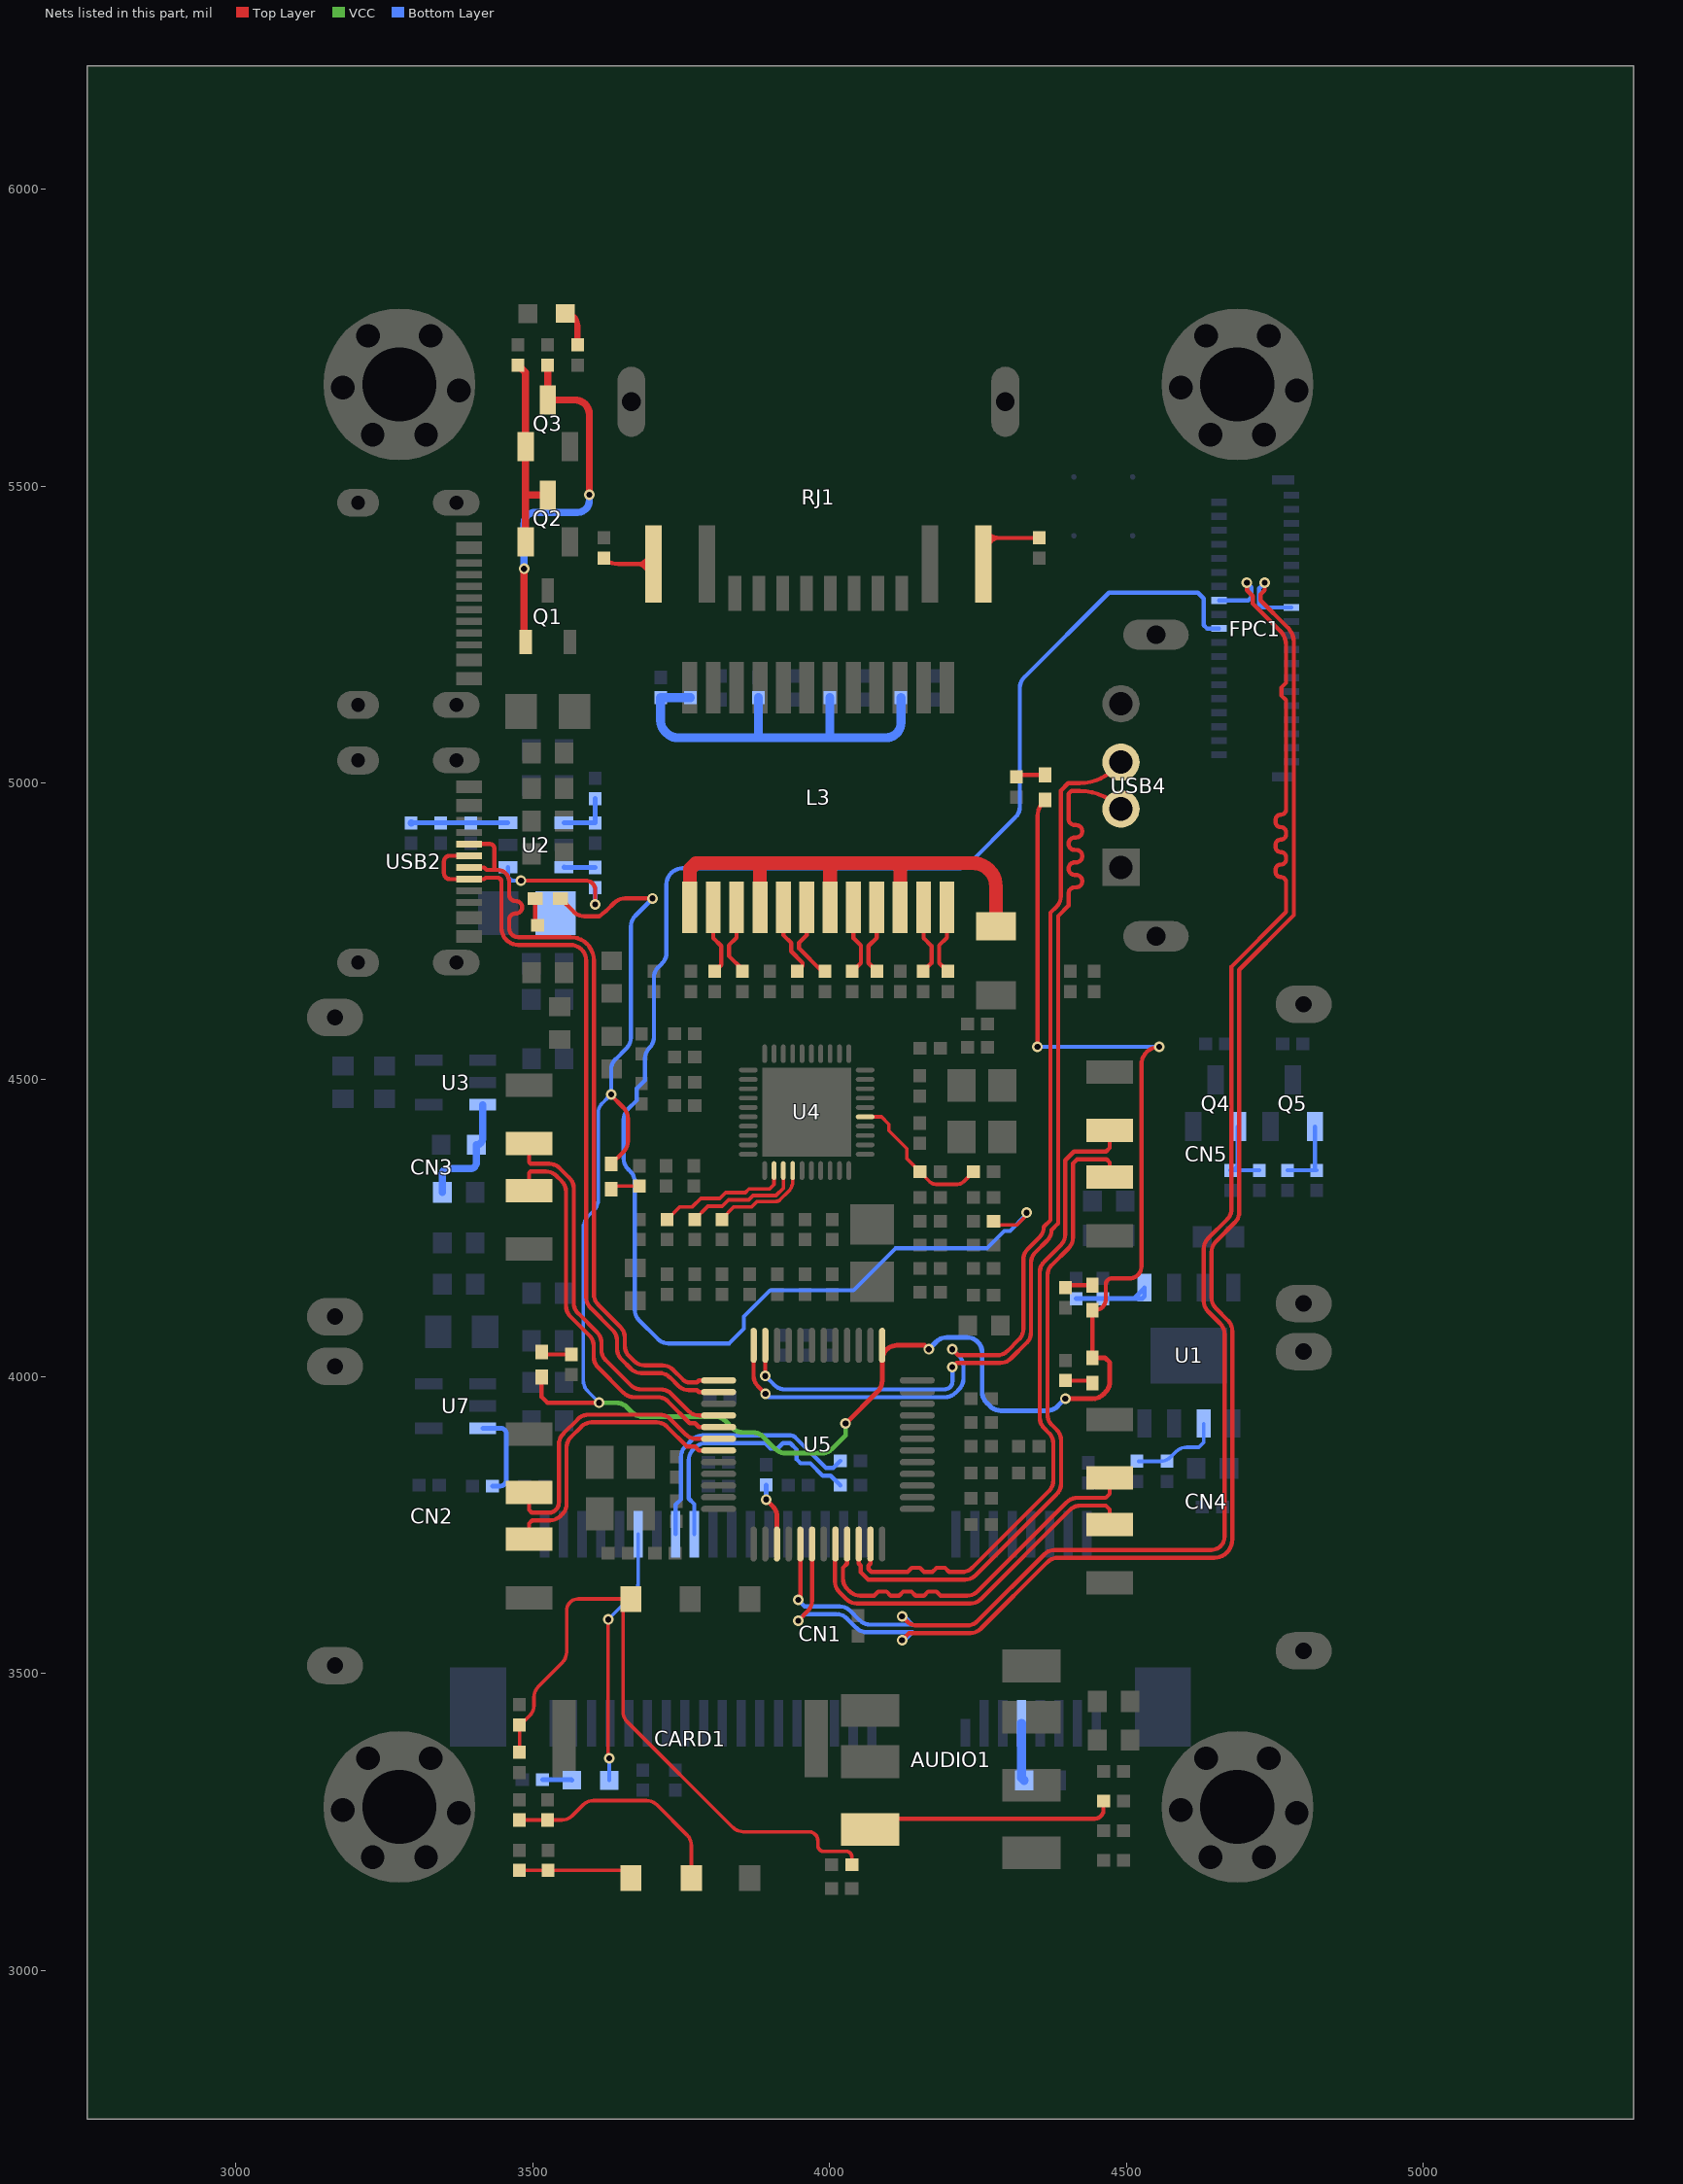
[diagram p0: the nets of this part, all layers, seen from the top]
# Altium PCB MISC84334.PcbDoc (part 4 of 8)
Units mil, origin at the board's own origin, x right, y up, seen from the top; angles counter-clockwise.
Board outline 2605.13 x 3457.4 mil, 4 copper layers (Top Layer, GND, VCC, Bottom Layer), stack 62.447 mil thick; 209 components, 149 nets, 735 pads, 529 vias.

## Via types
v1: diameter 18, hole 10, Top Layer to Bottom Layer, 529 vias

## Nets (pads, with @x,y where several pads share a name; then routed paths per layer and width w, separated by ;. In a path a pad name is that pad's centre, name@x,y a point inside that pad or via, vN(x,y) a via of type N, cw(c..) or ccw(c..) an arc to the next point about the centre after c; other vN are vias at no path point) (continued)
$2N2798: R45.1 U4.24 | length 168.6
  Top Layer w6: R45.1@3819.38,4264.89 3819.38,4266.28 3839.29,4286.19 3869.29,4286.19 3878.29,4295.19 3910.05,4295.19 ccw(c3910.05,4305.08) 3917.04,4298.09 3930.84,4311.88 ccw(c3913.16,4329.56) 3938.16,4329.56 U4.24@3938.16,4347.19
$2N2799: R46.1 U4.23 | length 200.8
  Top Layer w6: R46.1@3772.99,4264.89 3795.29,4287.19 3819.29,4287.19 3830,4297.9 3864,4297.9 3871.29,4305.19 3910.01,4305.19 3922.36,4317.54 U4.23@3922.36,4347.19
$2N2800: R48.1 U4.22 | length 228.1
  Top Layer w6: R48.1@3726.52,4264.89 3726.99,4264.89 3748.29,4286.19 3769.29,4286.19 3783.29,4300.19 3815.29,4300.19 3825.29,4310.19 3858.29,4310.19 3864.29,4316.19 3899.29,4316.19 3906.66,4323.56 U4.22@3906.66,4347.19
$2N2814: R23.1 R28.1 U4.35 | length 253.3
  Top Layer w6: U4.35@4060.16,4437.69 4087.79,4437.69 4100.29,4425.19 4100.29,4414.32 4130.29,4384.32 4130.29,4367.24 4169.11,4328.43 ccw(c4179.58,4338.9) 4179.58,4324.09 4215.64,4324.09 ccw(c4215.64,4338.35) 4225.73,4328.27 R23.1@4242.55,4345.09
$2N6665: R51.2 RJ1.12 | length 177.4
  Top Layer w7: RJ1.12@4259.39,5368.57 4259.39,5412.63 4285.36,5412.63 ; RJ1.12@4267.36,5420.09 ccw(c4285.36,5438.09) 4285.36,5412.63 ; RJ1.12@4268.79,5403.48 4272.7,5407.39 cw(c4285.36,5394.74) 4285.36,5412.63 ; R51.2@4353.17,5412.63 4285.36,5412.63
$2N6719: R47.2 RJ1.9 | length 132.6
  Top Layer w7: R47.2@3620.13,5378.55 ccw(c3644.22,5402.64) 3644.22,5368.57 3678.43,5368.57 ; RJ1.9@3695.84,5356.12 3686.9,5365.06 ccw(c3678.43,5356.58) 3678.43,5368.57 ; RJ1.9@3697.91,5382.25 3688.34,5372.68 cw(c3678.43,5382.59) 3678.43,5368.57 ; RJ1.9@3703.49,5368.57 3678.43,5368.57
$2N7042: C21.2 R37.1 R38.1 R39.1 R40.1 | length 701.2
  Bottom Layer w8: 3880.59,5076.51 3880.91,5076.19 ; 4000.59,5076.38 4000.78,5076.19
  Bottom Layer w15: R40.1@3765.59,5143.55 C21.2@3715.59,5143.55 3715.59,5104.69 ccw(c3740.59,5104.69) 3722.91,5087.01 3726.41,5083.51 ccw(c3744.09,5101.19) 3744.09,5076.19 3880.91,5076.19 4000.78,5076.19 4095.65,5076.19 ccw(c4095.65,5101.13) 4120.59,5101.13 R37.1@4120.59,5143.55 ; 3880.59,5076.51 R39.1@3880.59,5143.55 ; 4000.59,5076.38 R38.1@4000.59,5143.55
$2N7674: L3.2 R24.2 | length 118
  Top Layer w7: L3.2@3804.27,4790.55 3804.27,4738.76 3817.7,4725.34 3817.7,4693.42 R24.2@3806.91,4682.63
$2N7677: L3.3 R25.2 | length 122.6
  Top Layer w7: L3.3@3843.64,4790.55 3843.64,4739.38 3830.7,4726.44 3830.7,4708.65 3853.28,4686.07 R25.2@3853.28,4682.63
$2N7680: L3.5 R27.2 | length 125.2
  Top Layer w7: L3.5@3922.39,4790.55 3922.39,4743.74 3935.58,4730.56 3935.58,4716.36 3955.08,4696.85 3955.08,4691.69 R27.2@3946.02,4682.63
$2N7683: L3.6 R29.2 | length 134.1
  Top Layer w7: L3.6@3961.76,4790.55 3961.76,4743.74 3948.74,4730.72 3948.74,4721.58 3987.69,4682.63 R29.2@3992.38,4682.63
$2N7686: L3.8 R31.2 | length 118.9
  Top Layer w7: R31.2@4038.75,4682.63 4052.94,4696.81 4052.94,4726.33 4040.5,4738.76 L3.8@4040.5,4790.55
$2N7689: L3.9 R32.2 | length 119.6
  Top Layer w7: L3.9@4079.86,4790.55 4079.87,4739.38 4065.94,4725.45 4065.94,4696.81 R32.2@4080.12,4682.63
$2N7692: L3.12 R35.2 | length 119.2
  Top Layer w7: L3.12@4197.98,4790.55 4197.98,4739.38 4185.04,4726.44 4185.04,4696.81 R35.2@4199.22,4682.63
$2N7695: L3.11 R34.2 | length 119.4
  Top Layer w7: R34.2@4157.86,4682.63 4172.04,4696.81 4172.04,4725.34 4158.61,4738.76 L3.11@4158.61,4790.55
$2N7873: C20.2 L3.1 L3.4 L3.7 L3.10 | length 897.6
  Top Layer w15: 4000.66,4865.19 4001.13,4864.72 ; 4119.15,4865.19 4119.23,4865.11
  Top Layer w23: L3.1@3764.9,4790.55 3764.9,4854.8 3775.29,4865.19 3883.24,4865.19 ; L3.4@3883.02,4790.55 3883.02,4864.97 3883.24,4865.19 ; L3.7@4001.13,4790.55 4001.13,4864.72 ; 4119.15,4865.19 4000.66,4865.19 3883.24,4865.19 ; L3.10@4119.23,4790.55 4119.23,4865.11 4240.81,4865.11 cw(c4240.81,4825.33) 4280.59,4825.33 C20.2@4280.59,4758.81
$3N2816: CN1.42 LED8.1 | length 435.4
  Top Layer w6: v1(3627.29,3591.19) 3627.29,3358.95 v1(3629.05,3357.19)
  Bottom Layer w6: v1(3627.29,3591.19) 3670.54,3634.44 ccw(c3652.87,3652.12) 3677.87,3652.12 CN1.42@3677.87,3735.04 ; LED8.1@3629.05,3320.24 v1(3629.05,3357.19)
$3N2817: LED8.2 R70.1 | length 49.6
  Bottom Layer w8: R70.1@3516.74,3321.19 3565.42,3321.19 LED8.2@3566.1,3320.51
$3N2819: CN1.9 L7.2 | length 97.8
  Bottom Layer w15: CN1.9@4323.54,3416.14 4323.54,3324.73 L7.2@4328.04,3320.23
$3N2827: CN1.36 R68.1 | length 445.9
  Bottom Layer w7: CN1.36@3772.36,3735.04 3772.36,3785.64 3763.11,3794.89 3763.11,3859.65 cw(c3788.11,3859.65) 3770.43,3877.33 3773.97,3880.87 cw(c3791.65,3863.19) 3791.65,3888.19 3891.63,3888.19 3900.63,3879.19 3912.63,3879.19 3921.63,3888.19 3933.91,3888.19 3944.87,3877.23 3944.87,3860.61 3951.41,3854.07 3968.03,3854.07 3988.71,3833.38 4002.06,3833.38 R68.1@4018.25,3817.19
$3N2828: CN1.38 R69.1 | length 448
  Bottom Layer w7: CN1.38@3740.86,3735.04 3740.86,3784.51 3750.11,3793.76 3750.11,3865.04 cw(c3775.11,3865.04) 3757.43,3882.71 3768.58,3893.87 cw(c3786.26,3876.19) 3786.26,3901.19 3934.44,3901.19 cw(c3934.44,3889.47) 3942.72,3897.76 3994.1,3846.38 4006.44,3846.38 R69.1@4018.25,3858.19
$3N3897: CARD1.C2 D6.1 R63.2 | length 391.6
  Top Layer w6: R63.2@3477.77,3253.55 D6.1@3525.59,3253.55 3549.3,3253.55 ccw(c3549.3,3278.55) 3566.97,3260.87 3584.97,3278.87 cw(c3602.65,3261.19) 3602.65,3286.19 3691.94,3286.19 cw(c3691.94,3261.19) 3709.61,3278.87 3760.27,3228.21 cw(c3742.6,3210.53) 3767.6,3210.53 CARD1.C2@3767.6,3155.36
$3N3904: CARD1.C3 D5.1 R64.2 | length 193
  Top Layer w6: R64.2@3478.09,3168.55 D5.1@3525.8,3168.55 3652.4,3168.55 CARD1.C3@3665.6,3155.36
$3N4163: CARD1.C7 D8.1 R62.1 R65.1 | length 1097.8
  Top Layer w6: D8.1@3478.04,3367.63 R65.1@3478.04,3413.55 3479.65,3413.55 3494.97,3428.87 ccw(c3477.29,3446.55) 3502.29,3446.55 3502.29,3460.38 cw(c3527.29,3460.38) 3509.61,3478.06 3549.97,3518.41 ccw(c3532.29,3536.09) 3557.29,3536.09 3557.29,3606.19 cw(c3576.93,3606.19) 3576.93,3625.83 CARD1.C7@3665.6,3625.83 3652.29,3612.52 3652.29,3436.55 ccw(c3677.29,3436.55) 3659.61,3418.87 3837.47,3241.01 ccw(c3855.15,3258.69) 3855.15,3233.69 3965.41,3233.69 cw(c3965.41,3218.51) 3980.59,3218.51 3980.59,3210.59 ccw(c3990.59,3210.59) 3990.59,3200.59 4028.68,3200.59 cw(c4028.68,3191.5) 4037.77,3191.5 R62.1@4037.77,3177.96
$3N6344: C57.2 Q4.1 R66.2 | length 129.5
  Bottom Layer w7: Q4.1@4687.99,4421.22 4687.99,4360.03 cw(c4675.59,4360.03) R66.2@4675.59,4347.63 C57.2@4724.41,4347.63
$3N6376: C58.1 Q5.1 R72.1 | length 123.9
  Bottom Layer w7: R72.1@4771.77,4347.63 C58.1@4820.59,4347.63 cw(c4820.59,4350.23) 4817.99,4350.23 Q5.1@4817.99,4421.22
$4N635: AUDIO1.6 R75.2 | length 434.5
  Top Layer w7: AUDIO1.6@4068.8,3237.48 4068.8,3255.59 4446.61,3255.59 ccw(c4446.61,3270.59) 4461.61,3270.59 R75.2@4461.61,3285.59
$5N539: Q1.1 Q3.3 R6.2 | length 620.4
  Top Layer w12: v1(3485.59,5360.59) 3485.59,5239.83 Q1.1@3488.19,5237.23 ; R6.2@3525.59,5703.55 Q3.3@3525.59,5644.96 3571.22,5644.96 cw(c3571.22,5620.59) 3595.59,5620.59 v1(3595.59,5485.59)
  Bottom Layer w12: v1(3485.59,5360.59) 3485.59,5437.16 cw(c3504.02,5437.16) 3504.02,5455.59 3575.59,5455.59 ccw(c3575.59,5475.59) 3595.59,5475.59 v1(3595.59,5485.59)
$5N540: Q2.1 Q2.3 Q3.1 R5.2 | length 340.3
  Top Layer w12: R5.2@3475.59,5703.55 3488.19,5690.95 Q3.1@3488.19,5566.22 3488.19,5485.5 ; Q2.1@3488.19,5406.12 3488.19,5485.5 ; Q2.3@3525.59,5484.86 3488.82,5484.86 3488.19,5485.5
$5N1057: R2.1 R3.2 U1.5 | length 156.7
  Bottom Layer w8: R3.2@4415.59,4131.5 R2.1@4460.59,4131.5 4512.66,4131.5 ; U1.5@4530.59,4150.09 U1.5@4530.59,4149.43 ; 4512.66,4131.5 U1.5@4530.59,4149.43 ; 4512.66,4131.5 4526.8,4131.5 4530.59,4135.29 U1.5@4530.59,4149.43
$5N1555: R1.1 R4.2 U1.2 | length 152.6
  Bottom Layer w6: R4.2@4520.59,3857.63 4557.38,3857.63 ccw(c4557.38,3882.63) 4575.05,3864.95 4583.97,3873.87 cw(c4601.65,3856.19) 4601.65,3881.19 4622.29,3881.19 4630.59,3889.49 U1.2@4630.59,3921.09
$5N2255: R7.1 R9.2 U2.4 | length 93.6
  Bottom Layer w8: U2.4@3552.84,4932.99 R7.1@3605.23,4932.99 ; R7.1@3605.59,4932.63 R7.1@3605.23,4932.99 ; R9.2@3605.59,4973.55 3605.59,4933.35 R7.1@3605.23,4932.99
$5N2259: C6.2 U2.1 | length 227.3
  Top Layer w7: v1(3480.59,4835.59) 3589.34,4835.59 cw(c3589.34,4819.34) 3605.59,4819.34 v1(3605.59,4795.59)
  Bottom Layer w7: U2.1@3458.35,4858.19 3458.35,4844.68 ccw(c3467.43,4844.68) 3467.43,4835.59 v1(3480.59,4835.59) v1@3480.59,4835.95
  Bottom Layer w8: v1(3605.59,4795.59) C6.2@3605.59,4823.55
$5N2260: C6.1 L1.1 U2.6 | length 53.1
  Bottom Layer w8: U2.6@3552.84,4858.19 ccw(c3553.4,4858.19) 3553.4,4857.63 C6.1@3605.59,4857.63
$5N2261: C9.1 R8.1 R11.2 U2.3 | length 162.9
  Bottom Layer w8: R8.1@3295.95,4932.99 U2.3@3458.35,4932.99
  Bottom Layer w12: R8.1@3295.59,4932.63 R8.1@3295.95,4932.99
$5N2434: LED1.2 R10.1 | length 64.5
  Top Layer w10: LED1.2@3555.08,5790.47 cw(c3555.08,5769.96) 3575.59,5769.96 R10.1@3575.59,5737.63
$5N3813: C15.2 R12.2 U3.3 | length 202.8
  Bottom Layer w12: C15.2@3348.03,4310.59 3348.03,4341.15 cw(c3357.47,4341.15) 3357.47,4350.59 3395.59,4350.59 ccw(c3395.59,4360.25) 3405.25,4360.25 R12.2@3405.25,4390.59 ccw(c3405.25,4401.35) 3416.01,4401.35 U3.3@3416.01,4458.19
$6N3726: LED7.1 R57.1 | length 47
  Top Layer w7: R57.1@4397.83,4150.13 4401.98,4154.28 LED7.1@4443.09,4154.28
$6N3729: LED6.1 R56.1 | length 47
  Top Layer w7: R56.1@4397.83,3993.55 4438.94,3993.55 LED6.1@4443.09,3989.4
$6N3732: LED5.1 R55.1 | length 48.7
  Top Layer w7: R55.1@4315.33,5010.13 cw(c4323.99,5001.48) 4323.99,5013.72 LED5.1@4363.09,5013.72
$6N3735: LED4.1 R54.1 | length 47.4
  Top Layer w7: LED4.1@3504.4,4805.59 3504.4,4764.74 ccw(c3508.55,4764.74) R54.1@3508.55,4760.59
$6N3738: LED3.1 R53.1 | length 49
  Top Layer w6: LED3.1@3632.59,4316.9 3636.74,4321.05 R53.1@3679.83,4321.05
$6N3741: LED2.1 R52.1 | length 51.9
  Top Layer w6: LED2.1@3515.07,4041.78 3519.22,4037.63 R52.1@3565.22,4037.63
$6N3783: R58.1 U5.27 | length 106
  Top Layer w8: v1(3893.29,3793.19) 3904.37,3782.11 cw(c3886.69,3764.44) 3911.69,3764.44 U5.27@3911.69,3718.27
  Bottom Layer w8: v1(3893.29,3793.19) R58.1@3893.29,3817.7
$7N1407: R78.2 U7.3 | length 151.7
  Bottom Layer w8: U7.3@3416.01,3913.19 3446.77,3913.19 cw(c3446.77,3904.37) 3455.59,3904.37 3455.59,3825.78 cw(c3445.84,3825.78) 3445.84,3816.03 R78.2@3432.63,3816.03
DM1: CN2.2 U5.18 | length 497.7
  Top Layer w7: CN2.2@3493.98,3804.96 3493.98,3775.78 3498.57,3771.19 3529.32,3771.19 ccw(c3529.32,3783.19) 3537.81,3774.71 3540.27,3777.17 ccw(c3527.36,3788.12) 3544.29,3788.12 3544.29,3886.22 cw(c3569.29,3886.22) 3551.61,3903.9 3576.58,3928.87 cw(c3594.26,3911.19) 3594.26,3936.19 3714.19,3936.19 cw(c3714.19,3911.19) 3731.87,3928.87 3757.98,3902.75 ccw(c3775.66,3920.43) 3775.66,3895.43 U5.18@3813.27,3895.43
DM2: CN3.2 U5.16 | length 662.6
  Top Layer w7: CN3.2@3493.98,4392.46 3493.98,4361.07 3496.46,4358.59 3527.92,4358.59 cw(c3527.92,4333.59) 3545.6,4351.27 3561.97,4334.9 cw(c3544.29,4317.22) 3569.29,4317.22 3569.29,4124.55 ccw(c3594.29,4124.55) 3576.61,4106.87 3608.57,4074.92 cw(c3590.89,4057.24) 3615.89,4057.24 3615.89,4045.65 ccw(c3640.89,4045.65) 3623.21,4027.97 3665.15,3986.03 ccw(c3682.83,4003.71) 3682.83,3978.71 3715.8,3978.71 cw(c3715.8,3953.71) 3733.48,3971.39 3762.74,3942.12 ccw(c3780.42,3959.8) 3780.42,3934.8 U5.16@3813.27,3934.8
DM3: U5.13 USB2.5 USB2.7 | length 1296.2
  Top Layer w7: USB2.7@3393.1,4857.75 3418.35,4857.75 3422.52,4853.57 3435.35,4853.57 ; USB2.5@3393.1,4897.12 3428.16,4897.12 cw(c3428.16,4889.68) 3435.59,4889.68 3435.59,4853.81 cw(c3435.35,4853.81) 3435.35,4853.57 ; 3460.59,4833.59 3460.59,4811.59 ccw(c3471.09,4811.59) 3471.09,4801.09 3471.94,4801.09 cw(c3471.94,4790.59) 3471.94,4780.09 3471.09,4780.09 ccw(c3471.09,4769.59) 3460.59,4769.59 3460.59,4755.59 ccw(c3475.91,4755.59) 3475.91,4740.27 3563.91,4740.27 cw(c3563.91,4700.89) 3603.29,4700.89 3603.29,4138.93 ccw(c3628.29,4138.93) 3610.61,4121.25 3647.97,4083.9 cw(c3630.29,4066.22) 3655.29,4066.22 3655.29,4052.42 ccw(c3680.29,4052.42) 3662.61,4034.74 3670.84,4026.51 ccw(c3688.52,4044.19) 3688.52,4019.19 3718.94,4019.19 cw(c3718.94,3994.19) 3736.61,4011.87 3753.75,3994.74 ccw(c3763.93,4004.92) 3763.93,3990.52 3776.9,3990.52 3780.24,3993.86 U5.13@3813.27,3993.86 ; 3460.59,4833.69 ccw(c3440.71,4833.69) 3440.71,4853.57 3435.35,4853.57
DM4: U5.11 USB4.2 | length 1682.3
  Top Layer w7: v1(3892.01,4001.19) U5.11@3892.01,4052.91 ; v1(4207.29,4016.19) 4214.29,4023.19 4287.81,4023.19 ccw(c4287.81,4048.19) 4305.49,4030.51 4332.34,4057.37 ccw(c4314.67,4075.05) 4339.67,4075.05 4339.67,4191.83 cw(c4364.67,4191.83) 4346.99,4209.5 4366.97,4229.48 ccw(c4349.29,4247.16) 4374.29,4247.16 4385.46,4258.33 4385.46,4775.98 4402.79,4793.3 4402.79,4813.65 cw(c4413.29,4813.65) 4413.29,4824.15 4415.49,4824.15 ccw(c4415.49,4834.65) 4415.49,4845.15 4413.29,4845.15 cw(c4413.29,4855.65) 4413.29,4866.15 4415.49,4866.15 ccw(c4415.49,4876.65) 4415.49,4887.15 4413.29,4887.15 cw(c4413.29,4897.65) 4413.29,4908.15 4415.49,4908.15 ccw(c4415.49,4918.65) 4415.49,4929.15 4413.29,4929.15 cw(c4413.29,4939.65) 4402.79,4939.65 4402.79,4981.69 4407.69,4986.59 4421.53,4986.59 cw(c4421.53,4892.05) 4488.38,4958.9 USB4.2@4491.06,4956.23
  Bottom Layer w7: v1(3892.01,4001.19) 3907.19,3986.01 ccw(c3924.87,4003.69) 3924.87,3978.69 4193.91,3978.69 ccw(c4193.91,3992.07) 4207.29,3992.07 v1(4207.29,4016.19)
DM5: CN4.2 U5.32 | length 639.6
  Top Layer w7: U5.32@4010.12,3718.27 4009.51,3717.66 4009.51,3655.08 ccw(c4034.51,3655.08) 4016.83,3637.4 4028.64,3625.59 ccw(c4046.32,3643.27) 4046.32,3618.27 4237.4,3618.27 ccw(c4237.4,3643.27) 4255.07,3625.59 4405.23,3775.75 cw(c4422.91,3758.07) 4422.91,3783.07 4465.66,3783.07 4472.2,3776.53 CN4.2@4472.2,3751.01
DM6: CN5.2 U5.34 | length 1116.6
  Top Layer w7: U5.34@4049.49,3718.27 4049.49,3685.24 4052.83,3681.9 4052.83,3670.81 4065.45,3658.19 4228.48,3658.19 ccw(c4228.48,3683.19) 4246.16,3665.51 4382.97,3802.32 ccw(c4365.29,3820) 4390.29,3820 4390.29,3892.84 ccw(c4365.29,3892.84) 4382.97,3910.51 4374.61,3918.87 cw(c4392.29,3936.55) 4367.29,3936.55 4367.29,4170.45 cw(c4392.29,4170.45) 4374.61,4188.13 4402.97,4216.48 ccw(c4385.29,4234.16) 4410.29,4234.16 4410.29,4359.19 4417.29,4366.19 4466.95,4366.19 4472.2,4360.94 CN5.2@4472.2,4336.01
DMU: FPC1.24 U5.29 | length 2790.2
  Top Layer w7: v1(3947.29,3624.19) 3951.06,3627.96 U5.29@3951.06,3718.27 ; v1(4122.29,3596.19) 4129.97,3588.51 ccw(c4147.65,3606.19) 4147.65,3581.19 4231.94,3581.19 ccw(c4231.94,3606.19) 4249.61,3588.51 4361.97,3700.87 cw(c4379.65,3683.19) 4379.65,3708.19 4643.19,3708.19 ccw(c4643.19,3730.59) 4665.59,3730.59 4665.59,4071.85 ccw(c4640.59,4071.85) 4658.27,4089.53 4637.91,4109.88 cw(c4655.59,4127.56) 4630.59,4127.56 4630.59,4215.24 cw(c4655.59,4215.24) 4637.91,4232.91 4670.04,4265.04 ccw(c4652.36,4282.72) 4677.36,4282.72 4677.36,4690.75 4769.29,4782.68 4769.29,4832.64 ccw(c4760.38,4832.64) 4760.38,4841.56 cw(c4760.38,4850.47) 4751.47,4850.47 4751.47,4853.64 cw(c4760.38,4853.64) 4760.38,4862.56 ccw(c4760.38,4871.47) 4769.29,4871.47 4769.29,4874.64 ccw(c4760.38,4874.64) 4760.38,4883.56 cw(c4760.38,4892.47) 4751.47,4892.47 4751.47,4895.64 cw(c4760.38,4895.64) 4760.38,4904.56 ccw(c4760.38,4913.47) 4769.29,4913.47 4769.29,4916.64 ccw(c4760.38,4916.64) 4760.38,4925.56 cw(c4760.38,4934.47) 4751.47,4934.47 4751.47,4937.64 cw(c4760.38,4937.64) 4760.38,4946.56 ccw(c4760.38,4955.47) 4769.29,4955.47 4769.29,5139.5 4761.29,5147.5 4761.29,5160.5 4769.29,5168.5 4769.29,5231.45 ccw(c4733.93,5231.45) 4761.97,5253 ccw(c4733.93,5231.45) 4758.93,5256.46 4713.29,5302.1 4713.29,5314.69 4703.29,5324.69 v1(4703.29,5337.19)
  Bottom Layer w7: v1(3947.29,3624.19) 3958.29,3613.19 4017.32,3613.19 cw(c4017.32,3588.19) 4035,3605.87 4050.85,3590.01 ccw(c4068.53,3607.69) 4068.53,3582.69 4139.82,3582.69 4126.32,3596.19 v1(4122.29,3596.19) ; FPC1.24@4656.27,5307.33 4705.57,5307.33 4710.79,5312.55 4710.79,5329.69 v1(4703.29,5337.19)
DP1: CN2.3 U5.19 | length 498.2
  Top Layer w7: CN2.3@3493.98,3726.22 3493.98,3752.65 3499.52,3758.19 3529.32,3758.19 ccw(c3529.32,3783.19) 3547,3765.51 3549.97,3768.48 ccw(c3532.29,3786.16) 3557.29,3786.16 3557.29,3880.84 cw(c3582.29,3880.84) 3564.61,3898.51 3581.97,3915.87 cw(c3599.65,3898.19) 3599.65,3923.19 3708.8,3923.19 cw(c3708.8,3898.19) 3726.48,3915.87 3759.92,3882.43 3773.56,3882.43 3780.24,3875.75 U5.19@3813.27,3875.75
DP2: CN3.3 U5.17 | length 668.3
  Top Layer w7: CN3.3@3493.98,4313.72 3493.98,4343.12 3496.46,4345.59 3522.54,4345.59 cw(c3522.54,4320.59) 3540.21,4338.27 3548.97,4329.51 cw(c3531.29,4311.84) 3556.29,4311.84 3556.29,4119.17 ccw(c3581.29,4119.17) 3563.61,4101.49 3595.57,4069.53 cw(c3577.89,4051.86) 3602.89,4051.85 3602.89,4033.65 ccw(c3627.89,4033.65) 3610.21,4015.97 3653.15,3973.03 ccw(c3670.83,3990.71) 3670.83,3965.71 3710.41,3965.71 cw(c3710.41,3940.71) 3728.09,3958.39 3764.75,3921.73 3773.63,3921.73 3780.24,3915.12 U5.17@3813.27,3915.12
DP3: U5.14 USB2.6 USB2.8 | length 1303.2
  Top Layer w7: USB2.6@3393.1,4877.44 3360.59,4877.44 ccw(c3360.59,4867.44) 3350.59,4867.44 3350.59,4848.07 ccw(c3360.59,4848.07) 3360.59,4838.07 USB2.8@3393.1,4838.07 3418.25,4838.07 ; 3418.35,4838.07 3420.77,4840.49 3440.69,4840.49 cw(c3440.69,4833.59) 3447.59,4833.59 3447.59,4755.59 ccw(c3475.91,4755.59) 3475.91,4727.27 3563.91,4727.27 cw(c3563.91,4700.89) 3590.29,4700.89 3590.29,4133.55 ccw(c3615.29,4133.55) 3597.61,4115.87 3634.97,4078.51 cw(c3617.29,4060.84) 3642.29,4060.84 3642.29,4047.03 ccw(c3667.29,4047.03) 3649.61,4029.35 3665.45,4013.51 ccw(c3683.13,4031.19) 3683.13,4006.19 3713.55,4006.19 cw(c3713.55,3981.19) 3731.23,3998.87 3745.26,3984.84 ccw(c3762.94,4002.52) 3762.94,3977.52 3776.9,3977.52 3780.24,3974.17 U5.14@3813.27,3974.17
DP4: U5.12 USB4.3 | length 1690.4
  Top Layer w7: U5.12@3872.32,4052.91 3872.32,4001.52 ccw(c3897.32,4001.52) 3879.64,3983.84 v1(3892.29,3971.19) ; v1(4207.29,4046.19) 4217.29,4036.19 4282.42,4036.19 ccw(c4282.42,4061.19) 4300.1,4043.51 4319.34,4062.76 ccw(c4301.67,4080.43) 4326.67,4080.43 4326.67,4197.21 cw(c4351.67,4197.21) 4333.99,4214.89 4353.97,4234.87 ccw(c4336.29,4252.55) 4361.29,4252.55 4372.46,4263.72 4372.46,4781.36 4382.47,4791.37 ccw(c4364.79,4809.04) 4389.79,4809.04 4389.79,4987.07 4402.31,4999.59 4421.54,4999.59 ccw(c4421.54,5082.05) 4479.84,5023.74 USB4.3@4491.06,5034.97
  Bottom Layer w7: v1(3892.29,3971.19) 3897.79,3965.69 4194.82,3965.69 ccw(c4194.82,3990.69) 4212.5,3973.01 4218.47,3978.98 ccw(c4200.79,3996.66) 4225.79,3996.66 4225.79,4017.34 ccw(c4200.79,4017.34) 4218.47,4035.01 v1(4207.29,4046.19)
DP5: CN4.3 U5.33 | length 639.5
  Top Layer w7: U5.33@4029.8,3718.27 4029.8,3685.24 4022.8,3678.24 4022.8,3660.17 ccw(c4047.8,3660.17) 4030.12,3642.49 4034.03,3638.59 ccw(c4051.71,3656.27) 4051.71,3631.27 4075.29,3631.27 4082.29,3638.27 4096.29,3638.27 4103.29,3631.27 4117.29,3631.27 4124.29,3638.27 4138.29,3638.27 4145.29,3631.27 4159.29,3631.27 4166.29,3638.27 4180.29,3638.27 4187.29,3631.27 4232.01,3631.27 ccw(c4232.01,3656.27) 4249.69,3638.59 4399.85,3788.75 cw(c4417.53,3771.07) 4417.53,3796.07 4465.38,3796.07 4472.2,3802.89 CN4.3@4472.2,3829.75
DP6: CN5.3 U5.35 | length 1111.4
  Top Layer w7: U5.35@4069.17,3718.27 4069.17,3685.24 4065.83,3681.9 4065.83,3676.19 4070.83,3671.19 4131.59,3671.19 4138.59,3678.19 4152.59,3678.19 4159.59,3671.19 4173.59,3671.19 4180.59,3678.19 4194.59,3678.19 4201.59,3671.19 4223.1,3671.19 ccw(c4223.1,3696.19) 4240.78,3678.51 4369.97,3807.71 ccw(c4352.29,3825.38) 4377.29,3825.38 4377.29,3887.45 ccw(c4352.29,3887.45) 4369.97,3905.13 4361.61,3913.48 cw(c4379.29,3931.16) 4354.29,3931.16 4354.29,4175.84 cw(c4379.29,4175.84) 4361.61,4193.51 4389.97,4221.87 ccw(c4372.29,4239.55) 4397.29,4239.55 4397.29,4364.58 4411.91,4379.19 4465.88,4379.19 4472.2,4385.51 CN5.3@4472.2,4414.75
DPU: FPC1.23 U5.30 | length 2797.9
  Top Layer w7: v1(3947.29,3589.19) 3963.43,3605.33 ccw(c3945.75,3623.01) 3970.75,3623.01 U5.30@3970.75,3718.27 ; v1(4122.29,3556.19) 4134.29,3568.19 4237.32,3568.19 ccw(c4237.32,3593.19) 4255,3575.51 4367.35,3687.87 cw(c4385.03,3670.19) 4385.03,3695.19 4648.19,3695.19 ccw(c4648.19,3725.59) 4678.59,3725.59 4678.59,4077.24 ccw(c4653.59,4077.24) 4671.27,4094.91 4650.91,4115.27 cw(c4668.59,4132.95) 4643.59,4132.95 4643.59,4209.85 cw(c4668.59,4209.85) 4650.91,4227.53 4683.04,4259.65 ccw(c4665.36,4277.33) 4690.36,4277.33 4690.36,4685.36 4782.29,4777.29 4782.29,5236.84 ccw(c4746.93,5236.84) 4774.97,5258.38 ccw(c4746.93,5236.84) 4771.93,5261.84 4726.29,5307.48 4726.29,5317.69 4733.29,5324.69 v1(4733.29,5337.19)
  Bottom Layer w7: v1(3947.29,3589.19) 3958.29,3600.19 4011.94,3600.19 cw(c4011.94,3575.19) 4029.61,3592.87 4045.47,3577.01 ccw(c4063.15,3594.69) 4063.15,3569.69 4139.82,3569.69 4126.32,3556.19 v1(4122.29,3556.19) ; v1(4733.29,5337.19) 4723.79,5327.69 4723.79,5301.51 4729.78,5295.52 FPC1.23@4778.31,5295.52
DRV: LED2.2 LED3.2 LED4.2 LED5.2 LED6.2 LED7.2 U5.1 | length 3771.3
  Top Layer w7: LED2.2@3515.07,3999.4 3515.07,3966.11 3524.99,3956.19 v1(3612.29,3956.19) ; LED4.2@3546.78,4805.59 3569.46,4782.91 ccw(c3587.14,4800.59) 3587.14,4775.59 3612.26,4775.59 3622.57,4783.32 ccw(c3607.57,4803.32) 3625.25,4785.65 3637.87,4798.27 cw(c3655.55,4780.59) 3655.55,4805.59 v1@3700.59,4805.59 ; v1@3630.59,4475.59 3653.27,4452.91 cw(c3635.59,4435.24) 3660.59,4435.24 3660.59,4396.64 cw(c3635.59,4396.64) 3653.27,4378.96 LED3.2@3632.59,4358.28 ; v1(4350.59,4555.59) 4350.59,4943.57 ; 4350.59,4943.57 cw(c4387.43,4943.57) 4361.38,4969.63 LED5.2@4363.09,4971.34 ; LED6.2@4443.09,4031.78 LED7.2@4443.09,4111.9 4446.9,4111.9 ccw(c4446.9,4130.59) 4465.59,4130.59 4465.59,4155.59 cw(c4475.59,4155.59) 4475.59,4165.59 4505.59,4165.59 ccw(c4505.59,4185.59) 4525.59,4185.59 4525.59,4525.59 cw(c4555.59,4525.59) v1(4555.59,4555.59)
  Top Layer w8: v1(4027.29,3921.19) 4081.54,3975.44 ccw(c4063.86,3993.12) 4088.86,3993.12 4088.86,4027.91 cw(c4113.86,4027.91) 4113.86,4052.91 4160.57,4052.91 v1(4167.29,4046.19) ; v1(4397.29,3963.09) 4443.84,3963.09 ccw(c4443.84,3988.09) 4461.51,3970.41 4464.97,3973.87 ccw(c4447.29,3991.55) 4472.29,3991.55 4472.29,4023.89 4464.4,4031.78 LED6.2@4443.09,4031.78
  VCC w8: v1(3612.29,3956.19) 3640.94,3956.19 cw(c3640.94,3931.19) 3658.61,3948.87 3667.36,3940.12 ccw(c3685.04,3957.79) 3685.04,3932.79 3807.29,3932.79 cw(c3807.29,3907.79) 3824.96,3925.47 3836.92,3913.51 ccw(c3854.6,3931.19) 3854.6,3906.19 3870.76,3906.19 cw(c3870.76,3881.19) 3888.44,3898.87 3908.79,3878.51 ccw(c3926.47,3896.19) 3926.47,3871.19 3986.94,3871.19 ccw(c3986.94,3896.19) 4004.61,3878.51 4027.29,3901.19 v1(4027.29,3921.19)
  Bottom Layer w6: v1(3612.29,3956.19) 3592.91,3975.57 cw(c3610.59,3993.25) 3585.59,3993.25 3585.59,4251.77 cw(c3610.59,4251.77) 3592.91,4269.45 3603.27,4279.81 ccw(c3585.59,4297.48) 3610.59,4297.48 3610.59,4443.54 cw(c3635.59,4443.54) 3617.91,4461.21 3624.97,4468.27
  Bottom Layer w7: 3624.97,4468.27 ccw(c3607.29,4485.95) 3630.39,4476.38 ccw(c3607.29,4485.95) 3632.29,4485.95 3632.29,4516.94 cw(c3657.29,4516.94) 3639.61,4534.61 3658.27,4553.27 ccw(c3640.59,4570.95) 3665.59,4570.95 3665.59,4758.54 cw(c3690.59,4758.54) 3672.91,4776.21 v1(3702.29,4805.59) ; v1(4350.59,4555.59) v1@4550.59,4555.59
  Bottom Layer w8: v1(4167.29,4046.19) 4179.97,4058.87 cw(c4197.65,4041.19) 4197.65,4066.19 4231.94,4066.19 cw(c4231.94,4041.19) 4249.61,4058.87 4249.97,4058.51 cw(c4232.29,4040.84) 4257.29,4040.84 4257.29,3974.25 ccw(c4282.29,3974.25) 4264.61,3956.57 4270.95,3950.23 ccw(c4288.63,3967.91) 4288.63,3942.91 4366.75,3942.91 ccw(c4366.75,3967.91) 4384.43,3950.23 v1(4397.29,3963.09)
  other v1: 3632.29,4475.59
GMAC0_INT: FPC1.20 R33.2 | length 2924.1
  Top Layer w6: R33.2@4276.63,4262.09 4283.13,4255.59 4315.95,4255.59 4332.29,4271.93 v1(4332.29,4276.19)
  Bottom Layer w7: v1(4332.29,4276.19) 4332.29,4273.6 4304.28,4245.59 4294.38,4245.59 4264.98,4216.19 4111.19,4216.19 4040.59,4145.59 3900.33,4145.59 3855.99,4101.24 3855.99,4080.89 3831.29,4056.19 3728.65,4056.19 cw(c3728.65,4081.19) 3710.97,4063.51 3679.61,4094.87 cw(c3697.29,4112.55) 3672.29,4112.55 3672.29,4327.84 ccw(c3647.29,4327.84) 3664.97,4345.51 3660.65,4349.83 cw(c3678.33,4367.51) 3653.33,4367.51 3653.33,4432.98 cw(c3678.33,4432.98) 3660.65,4450.66 3675.59,4465.59 3675.59,4485.59 3689.29,4499.29 3689.29,4536.03 cw(c3714.29,4536.03) 3696.61,4553.71 3696.97,4554.07 ccw(c3679.29,4571.74) 3704.29,4571.74 3704.29,4671.84 cw(c3729.29,4671.84) 3711.61,4689.51 3718.19,4696.09 ccw(c3700.51,4713.77) 3725.51,4713.77 3725.51,4829.06 cw(c3752.65,4829.06) 3752.65,4856.19 4216.94,4856.19 ccw(c4216.94,4881.19) 4234.61,4863.51 4313.47,4942.37 ccw(c4295.79,4960.05) 4320.79,4960.05 4320.79,5160.17 cw(c4345.79,5160.17) 4328.11,5177.85 4470.85,5320.59 4620.59,5320.59 4630.59,5310.59 4630.59,5265.59 4636.09,5260.09 FPC1.20@4656.27,5260.08